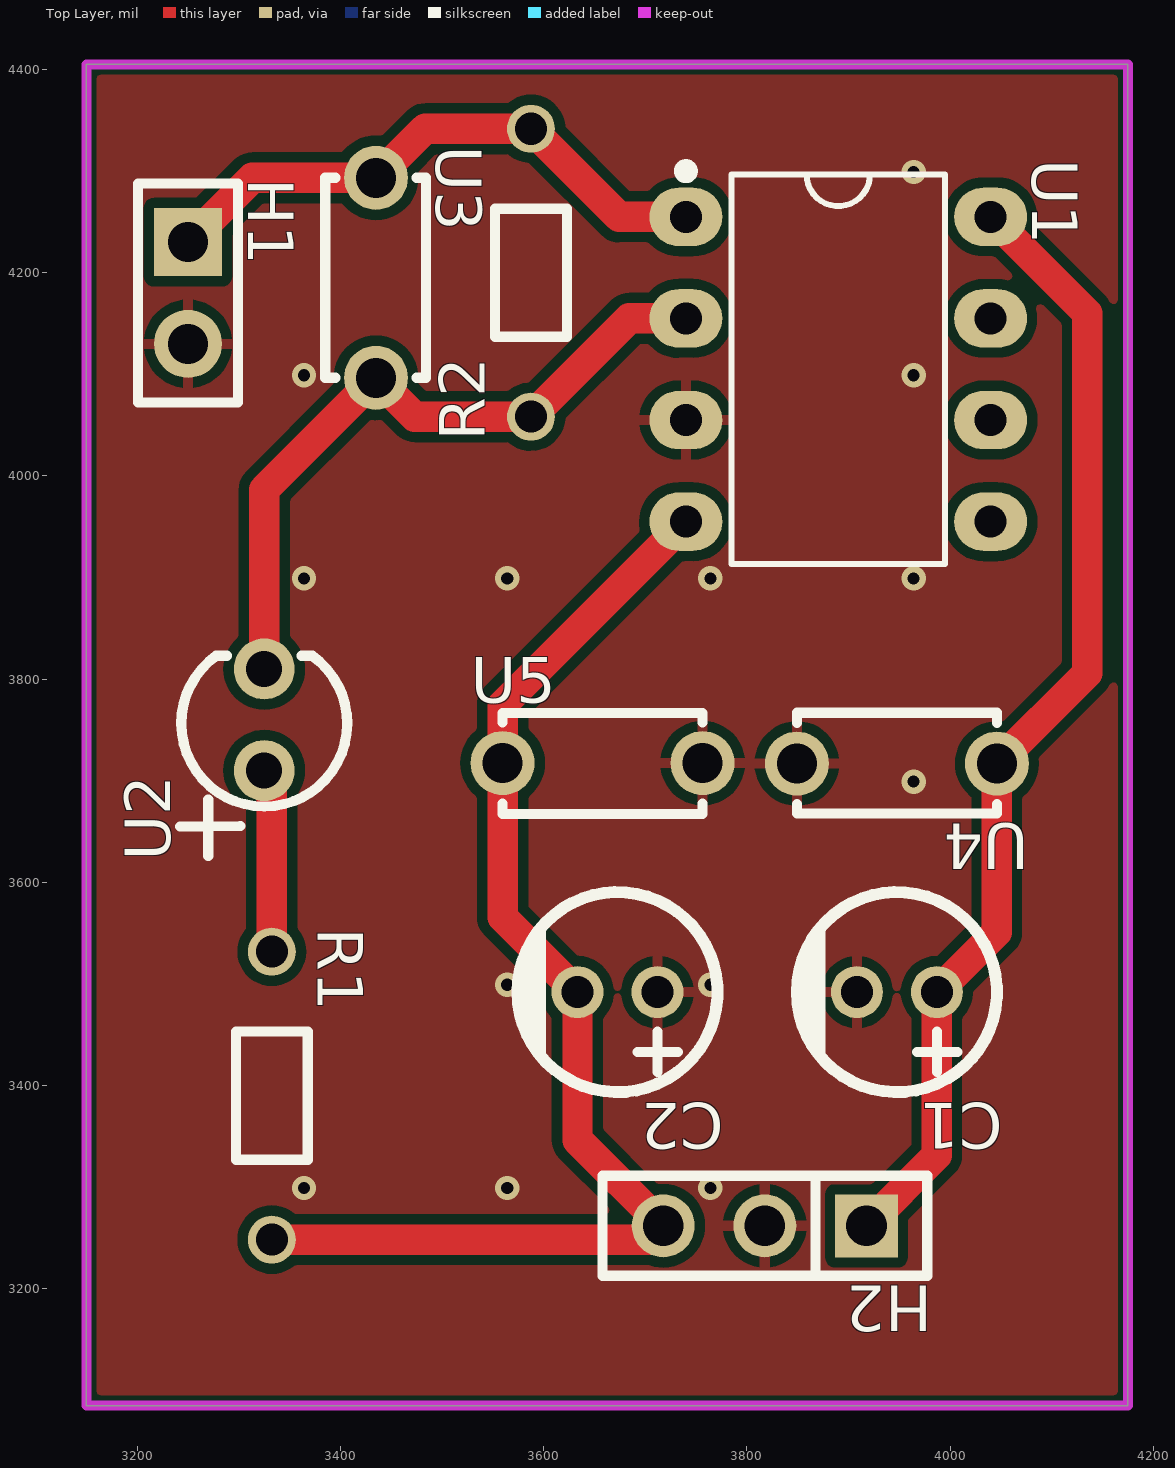
[diagram p0: Top Layer view]
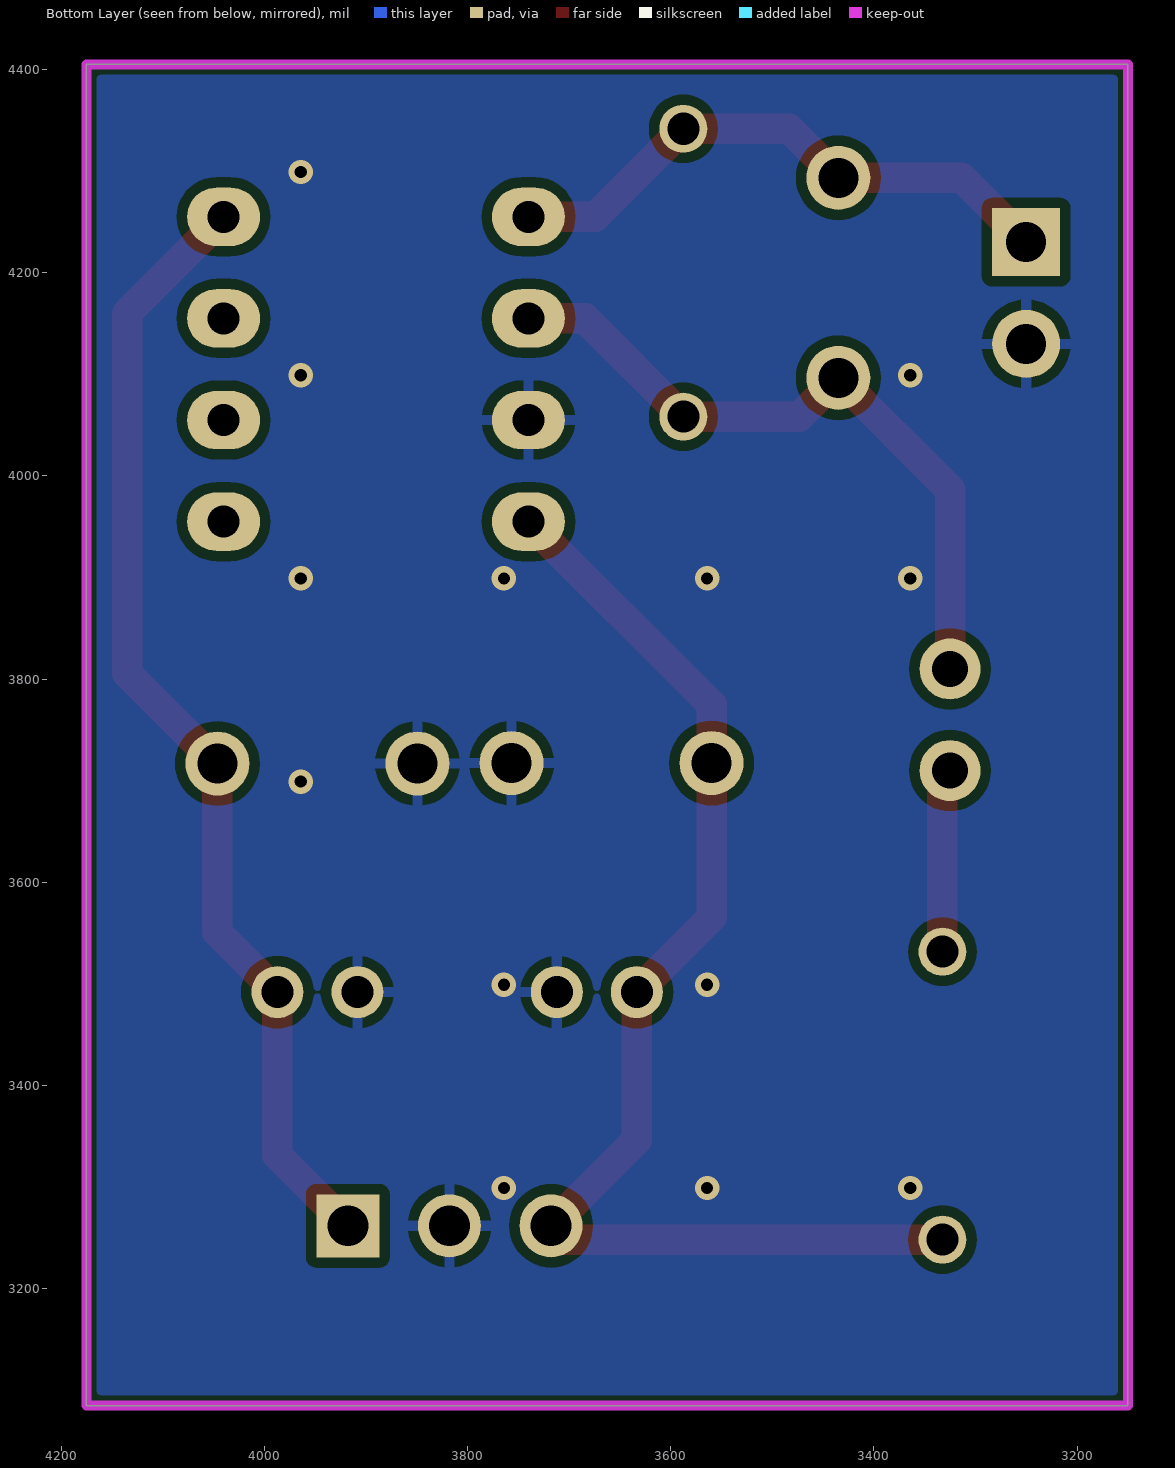
[diagram p1: Bottom Layer view, seen from below]
# Altium PCB MISC51879.pcbdoc
Units mil, origin at the board's own origin, x right, y up, seen from the top; angles counter-clockwise.
Board outline 1025 x 1320 mil, 2 copper layers (Top Layer, Bottom Layer), stack 62.206 mil thick; 11 components, 6 nets, 29 pads, 13 vias.

## Layer stack, top to bottom
Top Solder Mask Layer: solder mask 0.394, Dk 3.3
Top Layer: signal copper 1.379
Dielectric1: surface 59.449, FR4, Dk 4.5
Bottom Layer: signal copper 1.378
Bottom Solder Mask Layer: solder mask 0.394, Dk 3.3

## Board outline
3150,4405 3150,3085 4175,3085 4175,4405

## Design rules (kind name [scope] priority, off if disabled: settings)
BoardOutlineClearance copperThickness2oz_1 [All] p2 off: genericclearance=7.99 ignorepadtopadclearanceinfootprint=FALSE except(0: Arc-SplitContinuation Track-SplitContinuation SMDPad-SplitContinuation THPad-SplitContinuation Via-SplitContinuation Fill-SplitContinuation Region-SplitContinuation Poly-SplitContinuation Text-SplitContinuation Hole-SplitContinuation; 5.98: Arc-CutoutEdge SMDPad-CutoutEdge THPad-CutoutEdge Via-CutoutEdge Fill-CutoutEdge Region-CutoutEdge Text-CutoutEdge; 6.93: Hole-OutlineEdge Hole-CutoutEdge; 10: Poly-OutlineEdge Poly-CutoutEdge; 11.81: Arc-OutlineEdge Track-OutlineEdge SMDPad-OutlineEdge THPad-OutlineEdge Via-OutlineEdge Fill-OutlineEdge Region-OutlineEdge Text-OutlineEdge Track-CutoutEdge)
BoardOutlineClearance copperThickness1oz_1 [All] p4: genericclearance=4.02 ignorepadtopadclearanceinfootprint=FALSE except(0: Arc-SplitContinuation Track-SplitContinuation SMDPad-SplitContinuation THPad-SplitContinuation Via-SplitContinuation Fill-SplitContinuation Region-SplitContinuation Poly-SplitContinuation Text-SplitContinuation Hole-SplitContinuation; 6: SMDPad-CutoutEdge THPad-CutoutEdge Via-CutoutEdge Fill-CutoutEdge Region-CutoutEdge Text-CutoutEdge; 6.93: Hole-OutlineEdge Hole-CutoutEdge; 10: Poly-OutlineEdge Poly-CutoutEdge; 11.8: Arc-OutlineEdge Track-OutlineEdge SMDPad-OutlineEdge THPad-OutlineEdge Via-OutlineEdge Fill-OutlineEdge Region-OutlineEdge Text-OutlineEdge; 11.81: Arc-CutoutEdge Track-CutoutEdge)
Clearance copperThickness2oz [All] p1 off: gap=7.99 ignorepadtopadclearanceinfootprint=FALSE except(5.98: SMDPad-Track SMDPad-SMDPad THPad-Track SMDPad-THPad THPad-THPad Track-Via SMDPad-Via THPad-Via Via-Via Fill-Track Region-Track Fill-SMDPad Region-SMDPad Fill-THPad Region-THPad Fill-Via Region-Via Fill-Fill Fill-Region Region-Region Arc-Track Arc-SMDPad Arc-THPad Arc-Via Fill-Arc Region-Arc Arc-Arc Text-Track SMDPad-Text Text-THPad Text-Via Fill-Text Region-Text Arc-Text Text-Text; 6.93: Hole-Track Hole-SMDPad Hole-THPad Hole-Via Fill-Hole Region-Hole Hole-Arc Hole-Text; 10: Poly-Track Poly-SMDPad Poly-THPad Poly-Via Poly-Fill Poly-Region Poly-Poly Poly-Arc Poly-Text Poly-Hole)
Clearance copperThickness1oz [All] p3: gap=4.02 ignorepadtopadclearanceinfootprint=FALSE except(5.98: SMDPad-Track SMDPad-SMDPad THPad-Track SMDPad-THPad THPad-THPad Track-Via SMDPad-Via THPad-Via Via-Via Fill-Track Region-Track Fill-SMDPad Region-SMDPad Fill-THPad Region-THPad Fill-Via Region-Via Fill-Fill Fill-Region Region-Region; 6: Arc-Track Arc-SMDPad Arc-THPad Arc-Via Fill-Arc Region-Arc Arc-Arc Text-Track SMDPad-Text Text-THPad Text-Via Fill-Text Region-Text Arc-Text Text-Text; 6.93: Hole-Track Hole-SMDPad Hole-THPad Hole-Via Fill-Hole Region-Hole Hole-Arc Hole-Text; 10: Poly-Track Poly-SMDPad Poly-THPad Poly-Via Poly-Fill Poly-Region Poly-Poly Poly-Arc Poly-Text Poly-Hole)
Creepage creepage [All] p1: checkdistance=0 ignoreinternallayers=TRUE applytopolygonpour=TRUE
DiffPairsRouting differentialPair [All] p1: maxlimit=6 minlimit=6 mostfreqgap=6 toplayer_minwidth=5 toplayer_prefwidth=10 toplayer_maxwidth=100 toplayer_mingap=6 toplayer_prefgap=6 toplayer_maxgap=6 bottomlayer_minwidth=5 bottomlayer_prefwidth=10 bottomlayer_maxwidth=100 bottomlayer_mingap=6 bottomlayer_prefgap=6 bottomlayer_maxgap=6 maxuncoupledlength=10
HoleToHoleClearance otherClearance [All] p1: gap=11.81 allowstackedmicrovias=TRUE
Length netLength [All] p1: minlimit=0 maxlimit=0
MatchedLengths netLengthTolerance [All] p1: tolerance=1000
PasteMaskExpansion pasteMaskExpansion [All] p1: expansion=0
PlaneConnect innerPlane [All] p1: planeconnectstyle=Relief reliefexpansion=20 reliefentries=4 reliefconductorwidth=10 reliefairgap=10
PolygonConnect copperRegion [(InNet('GND'))] p1: connectstyle=Relief reliefconductorwidth=10 reliefentries=4 polygonreliefangle="90 Angle" airgapwidth=10 via.connectstyle=Relief via.reliefconductorwidth=10 via.reliefentries=4 via.polygonreliefangle="90 Angle" via.airgapwidth=10
RoutingVias viaSize [All] p1: holewidth=12.01 width=24.02 viastyle="Through Hole" minholewidth=11.81 minwidth=19.68 maxholewidth=248.03 maxwidth=393.7
SolderMaskExpansion solderMaskExpansion [IsVia] p1: expansion=-1000 istentingtop=TRUE
SolderMaskExpansion solderMaskExpansion [All] p2: expansion=2 istentingtop=FALSE
Width copperThickness2oz_2 [All] p1 off: maxlimit=100 minlimit=8 preferedwidth=10
Width copperThickness1oz_2 [All] p2: maxlimit=100 minlimit=5 preferedwidth=10

## Components (designator, comment, footprint, x,y, rotation, side; value= is the part's Value field where it differs from the comment)
C1 "10uF" CAP-TH_BD5.0-P2.00-D0.8-FD-10UF50VC110GL 3947.7,3491.91 r180 top
C2 "10uF" CAP-TH_BD5.0-P2.00-D0.8-FD-10UF50VC110GL 3672.7,3491.91 r180 top
H1 "" HDR-TH_2P-P2.54-V-F 3250,4180 r270 top
H2 "" HDR-TH_3P-P2.54-V-F 3817.7,3261.91 r180 top
R1 "100Ω" Res_1/8W 3330,3390 r270 top
R2 "100Ω" Res_1/8W 3590,4200 r90 top
U1 "NE5532P" DIP-8_L9.4-W6.4-P2.54-LS9.1-BL 3890,4105 r270 top
U2 "SFH 4356-UV" LED-TH_BD3.8-P2.54-FD 3325,3760 r90 top
U3 "2.2pF" CAP-TH_L5.0-W2.5-P5.00-D1.0 3435,4195 r270 top
U4 "100nF" CAP-TH_L5.0-W2.5-P5.00-D1.0 3947.7,3716.91 r180 top
U5 "100nF" CAP-TH_L5.0-W2.5-P5.00-D1.0 3658.09,3717.3 r0 top

## Footprints (in the part's own frame and the unit in brackets; to place one, negate y for a bottom-side part, rotate by r counter-clockwise, add the part's x,y. Pads: shape width x height; smd on the part's side, far side on the other; paste and mask are expansions set on the pad)
CAP-TH_BD5.0-P2.00-D0.8-FD-10UF50VC110GL [mm]
  round 1.3 hole 0.8: 1(-1,0) 2(1,0)
  silkscreen extent -2.5,-2.5 2.5,2.5
CAP-TH_L5.0-W2.5-P5.00-D1.0 [mm]
  round 1.6 hole 1: 1(-2.5,0) 2(2.5,0)
  silkscreen extent -2.5,-1.27 2.5,1.25
DIP-8_L9.4-W6.4-P2.54-LS9.1-BL [mm]
  oval 1.46x1.825 hole 0.8: 1(-3.81,-3.81) 2(-1.27,-3.81) 3(1.27,-3.81) 4(3.81,-3.81) 5(3.81,3.81) 6(1.27,3.81) 7(-1.27,3.81) 8(-3.81,3.81)
  silkscreen extent -5.1,-3.96 4.87,2.67
HDR-TH_2P-P2.54-V-F [mm]
  rect 1.7x1.7 hole 1: 1(-1.27,0)
  round 1.7 hole 1: 2(1.27,0)
  silkscreen extent -2.74,-1.25 2.74,1.25
HDR-TH_3P-P2.54-V-F [mil]
  rect 62x62 hole 40.16: 1(-100,0)
  round 62 hole 40.16: 2(0,0) 3(100,0)
  silkscreen extent -160,-49 160,49
LED-TH_BD3.8-P2.54-FD [mil]
  round 60 hole 35.43: 1(-50,0) 2(50,0)
  silkscreen extent -134,-82 63,83
Res_1/8W [mil]
  round 47.2 hole 31.5 paste+0 mask+2: 1(-141.7,2.48) 2(141.7,2.48)
  silkscreen extent -63,-33 63,38

## Via types
v1: diameter 24.02, hole 12, Top Layer to Bottom Layer, 13 vias

## Nets (pads, with @x,y where several pads share a name; then routed paths per layer and width w, separated by ;. In a path a pad name is that pad's centre, name@x,y a point inside that pad or via, vN(x,y) a via of type N, cw(c..) or ccw(c..) an arc to the next point about the centre after c; other vN are vias at no path point)
$1N80: R2.1 U1.2 U2.2 U3.2 | length 693
  Top Layer w30: U2.2 3325,3986.57 U3.2 3473.28,4058.3 R2.1 3684.22,4155 U1.2
$1N81: R1.1 U2.1 | length 181.4
  Top Layer w30: U2.1 3332.48,3702.52 R1.1
+5V: C1.1 H2.1 U1.8 U4.1 | length 1122.5
  Top Layer w30: H2.1 3987.07,3331.28 C1.1 4046.12,3550.96 U4.1 4135,3805.79 4135,4160 U1.8
-5V: C2.2 H2.3 R1.2 U1.4 U5.1 | length 1224.1
  Top Layer w30: R1.2 3704.09,3248.3 H2.3 3633.33,3346.28 C2.2 3559.67,3565.57 U5.1 3559.67,3774.67 U1.4
GND: C1.2 C2.1 H1.2 H2.2 U1.3 U4.2 U5.2
  other v1: 3364.1,3299.1 3564.1,3299.1 3764.1,3299.1 3564.1,3499.1 3764.1,3499.1 3964.1,3699.1 3364.1,3899.1 3564.1,3899.1 3764.1,3899.1 3964.1,3899.1 3364.1,4099.1 3964.1,4099.1 3964.1,4299.1
VOUT: H1.1 R2.2 U1.1 U3.1 | length 572.2
  Top Layer w30: H1.1 3313.43,4293.43 U3.1 3483.28,4341.7 R2.2 3674.22,4255 U1.1
pads on no net: U1.5 U1.6 U1.7

## Polygon pours and split planes (outlines as drawn)
GND on Top Layer (solid, remove dead copper, pour order 0): 3005,4495 3005,3000 4280,3000 4280,4495
GND on Bottom Layer (solid, remove dead copper, pour order 2): 3000,4445 3000,3065 4305,3065 4305,4445

## Keep-outs
Board Outline Layer:
  the board outline again, w10